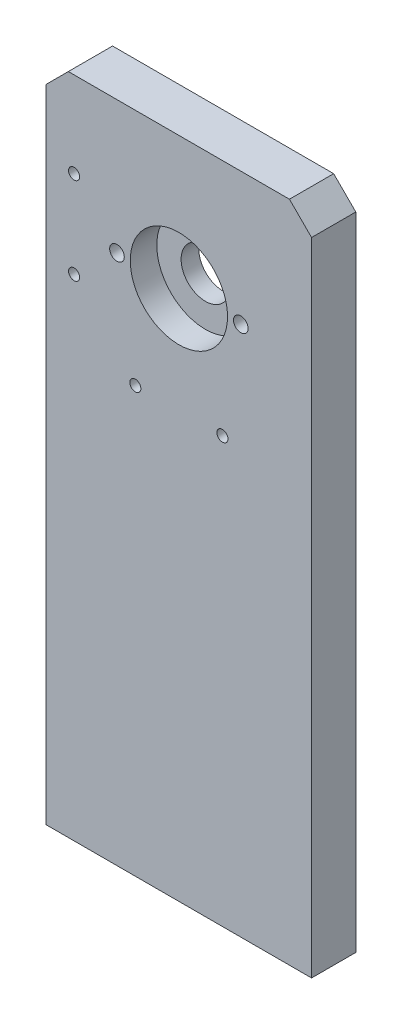
SolidWorks part; units mm, degrees
ref_plane "Front Plane" through (0, 0, 0) normal (0, 0, 1) x (1, 0, 0)
ref_plane "Top Plane" through (0, 0, 0) normal (0, 1, 0) x (1, 0, 0)
ref_plane "Right Plane" through (0, 0, 0) normal (1, 0, 0) x (0, 0, -1)
sketch "Sketch1" plane through (0, 0, 0) normal (0, 0, 1) x (1, 0, 0)
  line L1 (-30, 75) -> (30, 75)
  line L2 (-30, 75) -> (-30, -75)
  line L3 (-30, -75) -> (30, -75)
  line L4 (30, 75) -> (30, -75)
  line L5 (-30, 75) -> (30, -75) construction
  line L6 (-30, -75) -> (30, 75) construction
  point P0 (0, 0)
  dimension "D1" = 60
  dimension "D2" = 150
extrude "Boss-Extrude1" add sketch "Sketch1" along normal blind 10
chamfer "Chamfer1" distance 5 angle 45 2 edges at (30, 75, 5) (-30, 75, 5)
sketch "Sketch2" plane through (0, 0, 10) normal (0, 0, 1) x (1, 0, 0)
  line L0 (25, 75) -> (-25, 75) construction
  line L1 (0, 0) -> (0, 94.9227) construction
  circle A0 centre (0, 45) radius 11
  dimension "D1" = 22
  dimension "D2" = 30
extrude "Cut-Extrude1" cut sketch "Sketch2" against normal blind 6
sketch "Sketch3" plane through (0, 0, 4) normal (0, 0, 1) x (1, 0, 0)
  circle A0 centre (0, 45) radius 5.5
  dimension "D1" = 11
extrude "Cut-Extrude2" cut sketch "Sketch3" against normal through all
hole_wizard "M4 Tapped Hole1" positions "Sketch4" profile "Sketch5" tap size "M4" standard "GB" end condition through all
sketch "Sketch4" plane through (0, 0, 10) normal (0, 0, 1) x (1, 0, 0)
  line L0 (5.5, 45) -> (-37.5023, 45) construction
  line L3 (0, 39.5) -> (0, 63.1213) construction
  circle A0 centre (0, 45) radius 5.5 construction
  point P0 (-14, 45)
  point P17 (14, 45)
  dimension "D1" = 14
sketch "Sketch5" plane through (-14, 45, 10) normal (1, 0, 0) x (0, -1, 0)
  line L0 (0, 0) -> (0, 10)
  line L1 (0, 10) -> (1.65, 10)
  line L2 (1.65, 10) -> (1.65, 0)
  line L5 (1.65, 0) -> (0, 0)
  line L11 (0, -6.35) -> (0, 107.95) construction
  dimension "通孔螺纹孔钻头直径" = 3.3
  dimension "通孔螺纹孔钻头深度" = 10
cosmetic thread "Cosmetic Thread 1" parameters "D2"=4
cosmetic thread "Cosmetic Thread 2" parameters "D2"=4
hole_wizard "M4 Tapped Hole2" positions "Sketch7" profile "Sketch6" tap size "M4" standard "GB"
sketch "Sketch7" plane through (0, -75, 0) normal (0, -1, 0) x (-1, 0, 0)
  line L1 (20, -5) -> (-20, -5) construction
  line L2 (30, -10) -> (-30, -10) construction
  line L3 (30, 0) -> (-30, 0) construction
  line L4 (-30, -10) -> (-30, 0) construction
  line L5 (0, 0) -> (0, -5) construction
  point P9 (-20, -5)
  point P10 (20, -5)
  dimension "D1" = 10
sketch "Sketch6" plane through (-20, -75, 5) normal (1, 0, 0) x (0, 0, -1)
  line L0 (0, 0) -> (0, 12.4914)
  line L1 (0, 12.4914) -> (1.65, 11.5)
  line L2 (1.65, 11.5) -> (1.65, 0)
  line L5 (1.65, 0) -> (0, 0)
  line L10 (0, 12.4914) -> (-1.65, 11.5) construction
  line L11 (0, -6.35) -> (0, 107.95) construction
  dimension "螺纹孔钻头直径" = 3.3
  dimension "螺纹孔钻头深度" = 11.5
  dimension "导头角度" = 118
cosmetic thread "Cosmetic Thread 3" parameters "D1"=8, "D2"=4
cosmetic thread "Cosmetic Thread 4" parameters "D1"=8, "D2"=4
hole_wizard "M3 Tapped Hole1" positions "Sketch9" profile "Sketch8" tap size "M3" standard "GB" end condition through all
sketch "Sketch9" plane through (0, 0, 0) normal (0, 0, -1) x (-1, 0, 0)
  point P3 (-9.85, 21.1)
  point P10 (9.85, 21.1)
  point P17 (23.7, 35.95)
  point P24 (23.7, 55.65)
  dimension "D1" = 23.7
  dimension "D2" = 9.85
  dimension "D3" = 9.85
  dimension "D4" = 21.1
  dimension "D5" = 35.95
  dimension "D6" = 19.7
sketch "Sketch8" plane through (9.85, 21.1, 0) normal (1, 0, 0) x (0, 1, 0)
  line L0 (0, 0) -> (0, 10)
  line L1 (0, 10) -> (1.25, 10)
  line L2 (1.25, 10) -> (1.25, 0)
  line L5 (1.25, 0) -> (0, 0)
  line L11 (0, -6.35) -> (0, 107.95) construction
  dimension "通孔螺纹孔钻头直径" = 2.5
  dimension "通孔螺纹孔钻头深度" = 10
cosmetic thread "Cosmetic Thread 5" parameters "D2"=3
cosmetic thread "Cosmetic Thread 6" parameters "D2"=3
cosmetic thread "Cosmetic Thread 7" parameters "D2"=3
cosmetic thread "Cosmetic Thread 8" parameters "D2"=3
